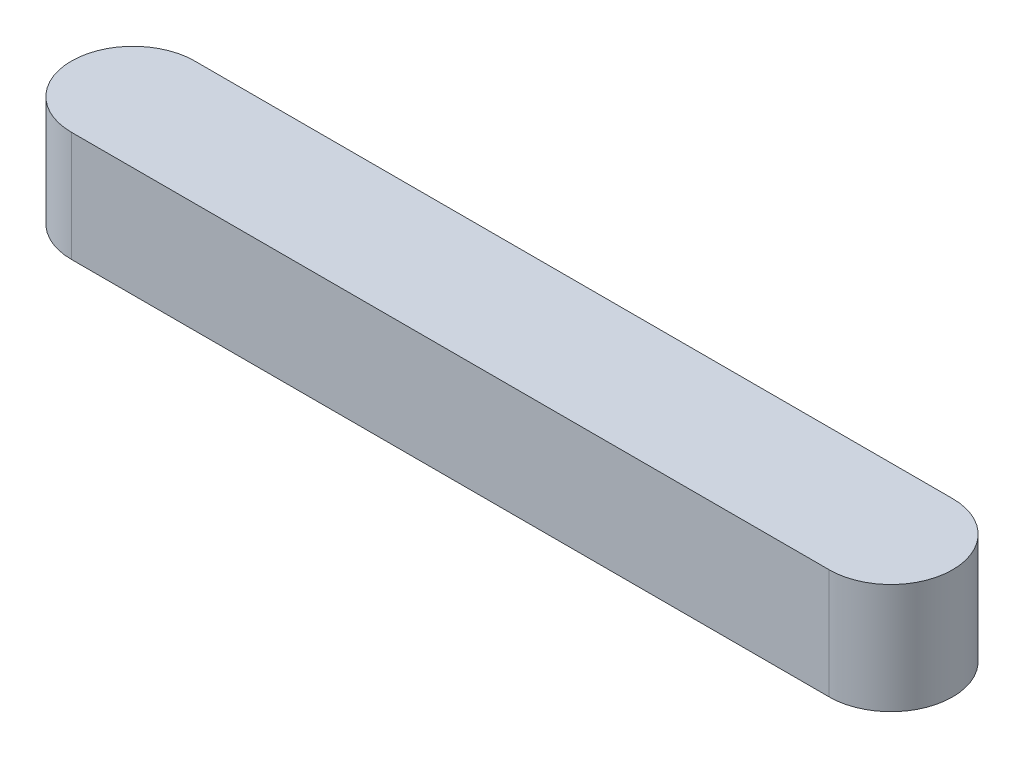
SolidWorks part; units mm, degrees
ref_plane "Front Plane" through (0, 0, 0) normal (0, 0, 1) x (1, 0, 0)
ref_plane "Top Plane" through (0, 0, 0) normal (0, 1, 0) x (1, 0, 0)
ref_plane "Right Plane" through (0, 0, 0) normal (1, 0, 0) x (0, 0, -1)
sketch "Sketch1" plane through (0, 0, 0) normal (0, 1, 0) x (1, 0, 0)
  line L0 (-75.6521, 0) -> (65.3269, 0) construction
  line L1 (-8.6, 1.4) -> (8.6, 1.4)
  line L2 (8.6, -1.4) -> (-8.6, -1.4)
  line L3 (0, 9.5065) -> (0, -7.1206) construction
  arc A0 (8.6, 1.4) -> (8.6, -1.4) centre (8.6, 0) cw
  arc A1 (-8.6, -1.4) -> (-8.6, 1.4) centre (-8.6, 0) cw
  dimension "D1" = 2.8
  dimension "D2" = 17.2
extrude "Boss-Extrude1" add sketch "Sketch1" along normal blind 2.5
